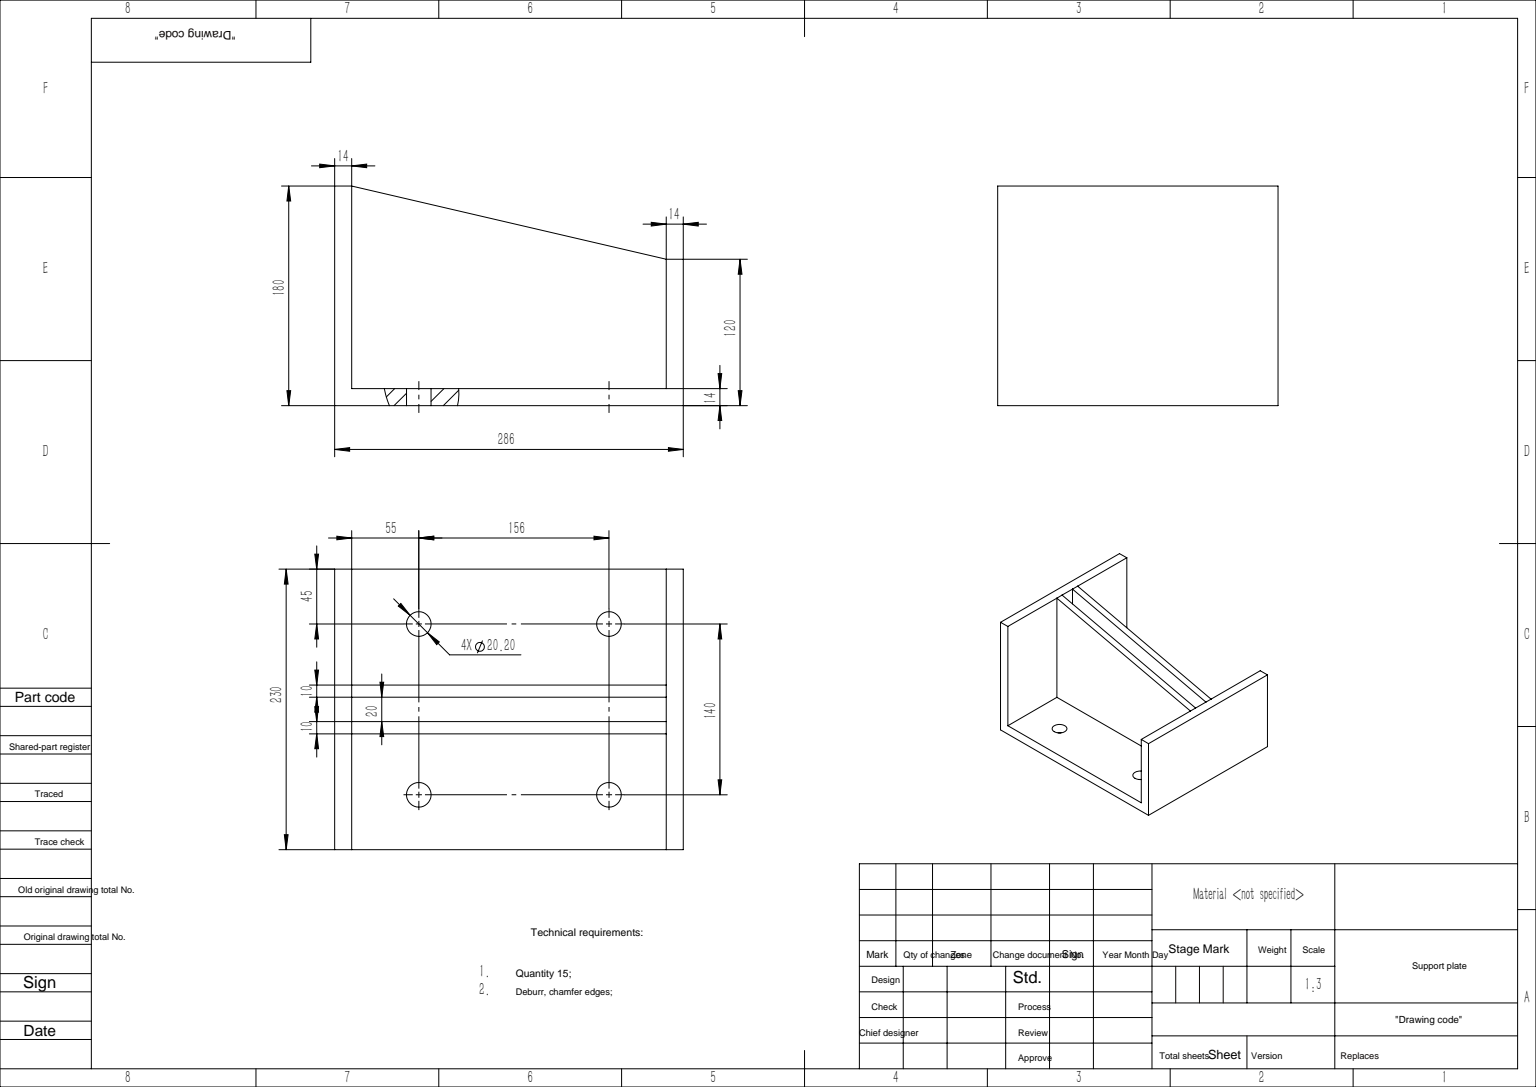
from build123d import *

# Parameters (mm, degrees)
EXTRUDE_1_DEPTH             = 115
EXTRUDE_START               = -10
EXTRUDE_2_DEPTH             = 10
EXTRUDE_START_2             = 10
EXTRUDE_3_DEPTH             = 10
SKETCH_4_R                  = 10.1
CUT_EXTRUDE_1_DEPTH         = 248.446964015
PATTERN_LINEAR_1_COUNT      = 2
PATTERN_LINEAR_1_PITCH      = 156
PATTERN_LINEAR_1_COUNT_DIR2 = 2
PATTERN_LINEAR_1_PITCH_DIR2 = 140


with BuildPart() as part:
    # 草图1 → 凸台-拉伸1 (new, symmetric)
    with BuildSketch(Plane.XY):
        Polygon((-143, 180), (-129, 180), (-129, 14), (129, 14), (129, 120), (143, 120), (143, 0), (-143, 0), align=None)
    extrude(amount=EXTRUDE_1_DEPTH, both=True)

    # 草图2 → 凸台-拉伸2 (add)
    with BuildSketch(Plane.XY.offset(EXTRUDE_START)):
        Polygon((129, 120), (129, 14), (-129, 14), (-129, 180), align=None)
    extrude(amount=-EXTRUDE_2_DEPTH)

    # 草图3 → 凸台-拉伸3 (add)
    with BuildSketch(Plane.XY.offset(EXTRUDE_START_2)):
        Polygon((-129, 180), (-129, 14), (129, 14), (129, 120), align=None)
    extrude(amount=EXTRUDE_3_DEPTH)

    # 草图4 → 切除-拉伸1 (cut, through all)
    with BuildSketch(Plane(origin=(0, 14, 0), x_dir=(1, 0, 0), z_dir=(0, 1, 0))):
        with Locations(Location((-74, -70, 0), (0, 0, 270))):
            Circle(SKETCH_4_R)
    cut_extrude_1 = extrude(amount=-CUT_EXTRUDE_1_DEPTH, mode=Mode.SUBTRACT)

    # 阵列(线性)1: Cut-Extrude 1 2 × 2
    with Locations(*[(i * PATTERN_LINEAR_1_PITCH, 0, -j * PATTERN_LINEAR_1_PITCH_DIR2) for i in range(PATTERN_LINEAR_1_COUNT) for j in range(PATTERN_LINEAR_1_COUNT_DIR2) if (i, j) != (0, 0)]):
        add(cut_extrude_1, mode=Mode.SUBTRACT)


solid = part.part
